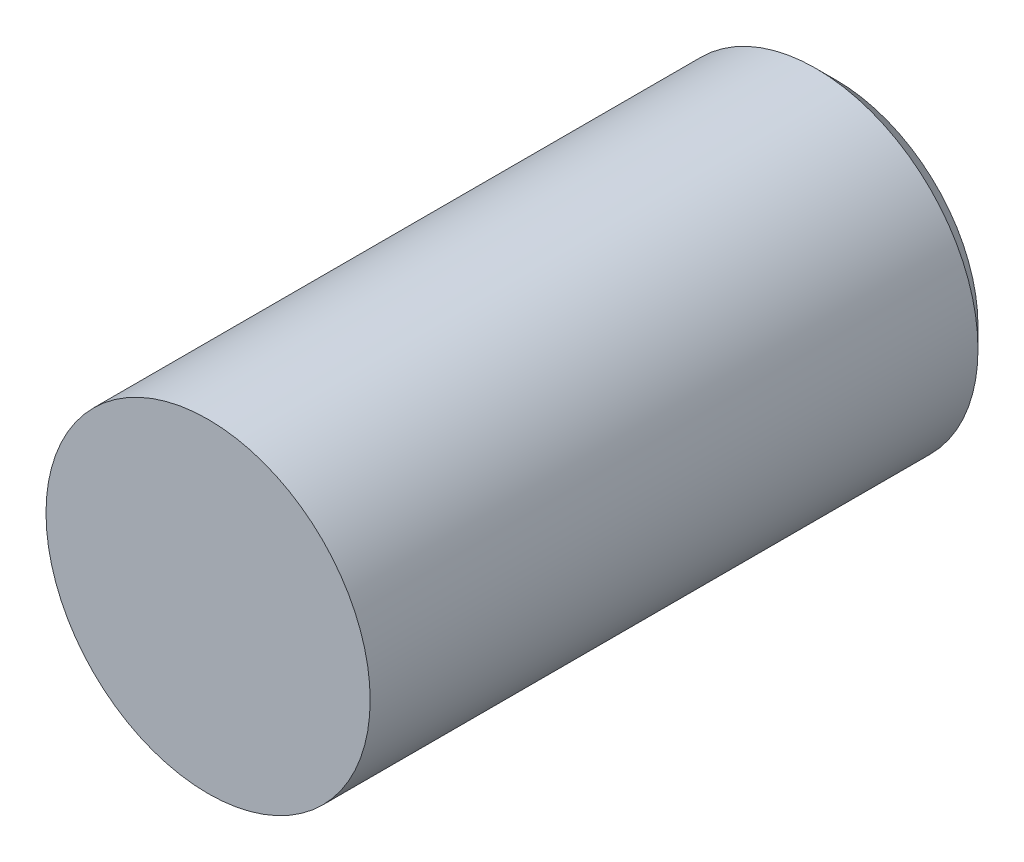
SolidWorks part; units mm, degrees
ref_plane "Front Plane" through (0, 0, 0) normal (0, 0, 1) x (1, 0, 0)
ref_plane "Top Plane" through (0, 0, 0) normal (0, 1, 0) x (1, 0, 0)
ref_plane "Right Plane" through (0, 0, 0) normal (1, 0, 0) x (0, 0, -1)
sketch "Sketch1" plane through (0, 0, 0) normal (0, 0, 1) x (1, 0, 0)
  circle A0 centre (0, 0) radius 8
  dimension "D1" = 16
extrude "Boss-Extrude1" add sketch "Sketch1" along normal blind 31
cosmetic thread "Cosmetic Thread1" parameters "D1"=10, "D2"=13.835
chamfer "Chamfer2" distance 1 angle 45 1 edges at (8, 0, 0)
